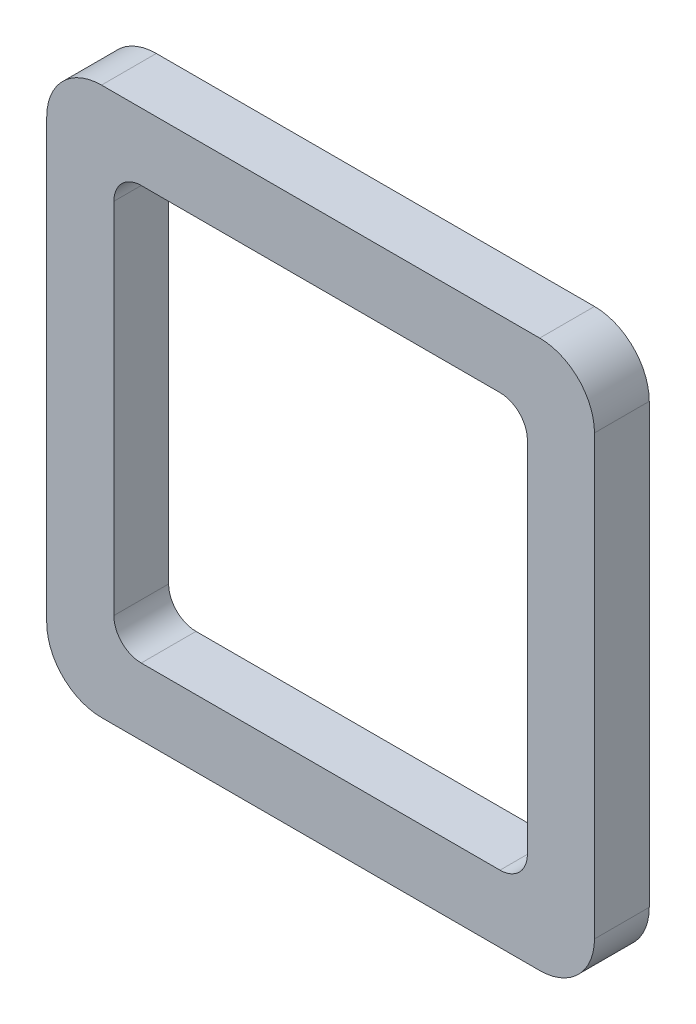
from build123d import *

# Parameters (mm, degrees)
SKETCH1_W           = 200
SKETCH1_H           = 200
SKETCH1_W_2         = 151
SKETCH1_H_2         = 151
BOSS_EXTRUDE1_DEPTH = 20
FILLET1_R           = 20
FILLET2_R           = 10


with BuildPart() as part:
    # Sketch1 → Boss-Extrude1 (new body)
    with BuildSketch(Plane.XY):
        with Locations((100, 100)):
            Rectangle(SKETCH1_W, SKETCH1_H)
        with Locations((100, 100)):
            Rectangle(SKETCH1_W_2, SKETCH1_H_2, mode=Mode.SUBTRACT)
    extrude(amount=BOSS_EXTRUDE1_DEPTH)

    # Fillet1
    fillet1_edges = [part.edges().sort_by_distance(p)[0] for p in [
        (0, 200, 10),
        (200, 200, 10),
        (200, 0, 10),
        (0, 0, 10),
    ]]
    fillet(fillet1_edges, radius=FILLET1_R)

    # Fillet2
    fillet2_edges = [part.edges().sort_by_distance(p)[0] for p in [
        (24.5, 175.5, 10),
        (24.5, 24.5, 10),
        (175.5, 24.5, 10),
        (175.5, 175.5, 10),
    ]]
    fillet(fillet2_edges, radius=FILLET2_R)


solid = part.part
